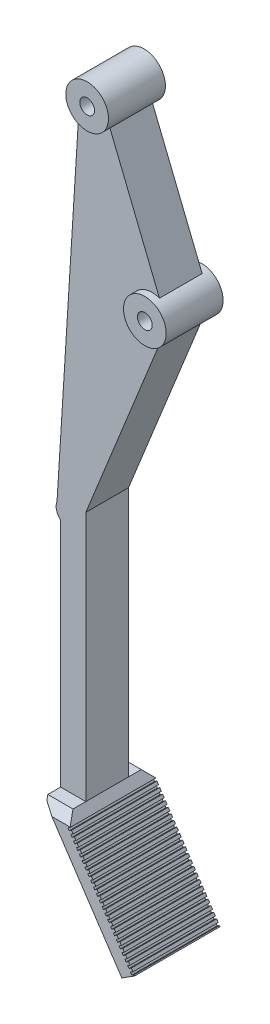
from build123d import *

# Parameters (mm, degrees)
SKETCH1_R            = 7.5
BOSS_EXTRUDE1_DEPTH  = 10
BOSS_EXTRUDE2_DEPTH  = 7.5
SKETCH3_R            = 2.6
CUT_EXTRUDE1_DEPTH   = 69.367154188
BOSS_EXTRUDE3_DEPTH  = 7.5
SKETCH6_R            = 7.5
BOSS_EXTRUDE4_DEPTH  = 10
SKETCH7_R            = 2.6
CUT_EXTRUDE2_DEPTH   = 139.291550533
BOSS_EXTRUDE8_DEPTH  = 7.5
SKETCH16_W           = 8.835752036
SKETCH16_H           = 88
BOSS_EXTRUDE9_DEPTH  = 7.5
BOSS_EXTRUDE10_DEPTH = 15
CHAMFER1_SIZE        = 3
CHAMFER2_SIZE        = 2
CUT_EXTRUDE3_DEPTH   = 259.435923483


with BuildPart() as part:
    # Sketch1 → Boss-Extrude1 (new, symmetric)
    with BuildSketch(Plane.XY):
        Circle(SKETCH1_R)
    extrude(amount=BOSS_EXTRUDE1_DEPTH, both=True)

    # Sketch2 → Boss-Extrude2 (add, symmetric)
    with BuildSketch(Plane.XY):
        with BuildLine():
            Line((5.502792208, -5.096006075), (24.97443042, -53.29000183))
            ThreePointArc((24.97443042, -53.29000183), (22.170934791, -59.894623641), (15.566312979, -57.091128012))
            Line((15.566312979, -57.091128012), (-5.395048503, -5.209937778))
            ThreePointArc((-5.395048503, -5.209937778), (0.078404622, -7.49959017), (5.502792208, -5.096006075))
        make_face()
    extrude(amount=BOSS_EXTRUDE2_DEPTH, both=True)

    # Sketch3 → Cut-Extrude1 (cut, through all)
    with BuildSketch(Plane.XY.offset(10)):
        Circle(SKETCH3_R)
    extrude(amount=-CUT_EXTRUDE1_DEPTH, mode=Mode.SUBTRACT)

    # Sketch5 → Boss-Extrude3 (add, symmetric)
    with BuildSketch(Plane.XY):
        with BuildLine():
            Line((15.566312979, -57.091128012), (-13.08078666, -127.995187718))
            ThreePointArc((-13.08078666, -127.995187718), (-10.670876789, -133.672579589), (-4.993484918, -131.262669718))
            Line((-4.993484918, -131.262669718), (24.944176558, -57.164357377))
            ThreePointArc((24.944176558, -57.164357377), (20.230755301, -60.263901008), (15.566312979, -57.091128012))
        make_face()
    extrude(amount=BOSS_EXTRUDE3_DEPTH, both=True)

    # Sketch6 → Boss-Extrude4 (add, symmetric)
    with BuildSketch(Plane.XY):
        with Locations((20.2703717, -55.190564921)):
            Circle(SKETCH6_R)
    extrude(amount=BOSS_EXTRUDE4_DEPTH, both=True)

    # Sketch7 → Cut-Extrude2 (cut, through all)
    with BuildSketch(Plane.XY.offset(10)):
        with Locations((20.2703717, -55.190564921)):
            Circle(SKETCH7_R)
    extrude(amount=-CUT_EXTRUDE2_DEPTH, mode=Mode.SUBTRACT)

    # Sketch11 → Boss-Extrude8 (add, symmetric)
    with BuildSketch(Plane.XY):
        with BuildLine():
            Line((-5.395048503, -5.209937778), (-13.08078666, -127.995187718))
            Line((-13.08078666, -127.995187718), (14.432076042, -59.898462945))
            ThreePointArc((14.432076042, -59.898462945), (12.821975428, -56.068854724), (13.497151784, -51.969774339))
            Line((13.497151784, -51.969774339), (-5.395048503, -5.209937778))
        make_face()
    extrude(amount=BOSS_EXTRUDE8_DEPTH, both=True)

    # Sketch16 → Boss-Extrude9 (add, symmetric)
    with BuildSketch(Plane.XY):
        with Locations((-7.390806842, -170.261622843)):
            Rectangle(SKETCH16_W, SKETCH16_H)
    extrude(amount=BOSS_EXTRUDE9_DEPTH, both=True)

    # Sketch17 → Boss-Extrude10 (add, symmetric)
    with BuildSketch(Plane(origin=(0, 0, 0), x_dir=(-1, 0, 0), z_dir=(0, 0, -1))):
        Polygon((11.80868286, -214.261622843), (2.972930824, -214.261622843), (-21.695736326, -251.232618801), (-15.495288767, -255.182156512), align=None)
    extrude(amount=BOSS_EXTRUDE10_DEPTH, both=True)

    # Chamfer1
    chamfer1_edges = [part.edges().sort_by_distance(p)[0] for p in [
        (-7.390806842, -214.261622843, 15),
        (-7.390806842, -214.261622843, -15),
    ]]
    chamfer(chamfer1_edges, length=CHAMFER1_SIZE)

    # Chamfer2
    chamfer2_edges = [part.edges().sort_by_distance(p)[0] for p in [
        (2.844168626, -236.221889677, 15),
        (2.844168626, -236.221889677, -15),
    ]]
    chamfer(chamfer2_edges, length=CHAMFER2_SIZE)

    # Sketch18 → Cut-Extrude3 (cut, through all)
    with BuildSketch(Plane.XY.offset(15)):
        Polygon((-0.922260896, -217.334967226), (-0.478234895, -218.000430155), (-1.310063556, -218.555462656), (-1.754089558, -217.889999727), align=None)
        Polygon((-0.755031055, -219.387291318), (0.076797607, -218.832258816), (0.520823608, -219.497721745), (-0.311005053, -220.052754247), align=None)
        Polygon((0.244027448, -220.884582909), (1.07585611, -220.329550407), (1.519882111, -220.995013336), (0.68805345, -221.550045838), align=None)
        Polygon((1.243085951, -222.381874499), (2.074914613, -221.826841998), (2.518940614, -222.492304927), (1.687111953, -223.047337429), align=None)
        Polygon((2.242144454, -223.87916609), (3.073973116, -223.324133588), (3.517999117, -223.989596518), (2.686170456, -224.544629019), align=None)
        Polygon((3.241202957, -225.376457681), (4.073031619, -224.821425179), (4.51705762, -225.486888108), (3.685228959, -226.04192061), align=None)
        Polygon((4.24026146, -226.873749271), (5.072090122, -226.31871677), (5.516116123, -226.984179699), (4.684287462, -227.539212201), align=None)
        Polygon((5.239319963, -228.371040862), (6.071148625, -227.81600836), (6.515174626, -228.48147129), (5.683345965, -229.036503791), align=None)
        Polygon((6.238378466, -229.868332453), (7.070207128, -229.313299951), (7.514233129, -229.97876288), (6.682404468, -230.533795382), align=None)
        Polygon((7.237436969, -231.365624043), (8.069265631, -230.810591542), (8.513291632, -231.476054471), (7.681462971, -232.031086973), align=None)
        Polygon((8.236495472, -232.862915634), (9.068324134, -232.307883132), (9.512350135, -232.973346062), (8.680521474, -233.528378563), align=None)
        Polygon((9.235553975, -234.360207225), (10.067382637, -233.805174723), (10.511408638, -234.470637652), (9.679579977, -235.025670154), align=None)
        Polygon((10.234612478, -235.857498816), (11.06644114, -235.302466314), (11.510467141, -235.967929243), (10.67863848, -236.522961745), align=None)
        Polygon((11.233670981, -237.354790406), (12.065499643, -236.799757905), (12.509525644, -237.465220834), (11.677696983, -238.020253335), align=None)
        Polygon((12.232729484, -238.852081997), (13.064558146, -238.297049495), (13.508584147, -238.962512424), (12.676755486, -239.517544926), align=None)
        Polygon((13.231787987, -240.349373588), (14.063616649, -239.794341086), (14.50764265, -240.459804015), (13.675813989, -241.014836517), align=None)
        Polygon((14.23084649, -241.846665178), (15.062675152, -241.291632677), (15.506701153, -241.957095606), (14.674872492, -242.512128108), align=None)
        Polygon((15.229904993, -243.343956769), (16.061733655, -242.788924267), (16.505759656, -243.454387197), (15.673930995, -244.009419698), align=None)
        Polygon((16.228963496, -244.84124836), (17.060792158, -244.286215858), (17.504818159, -244.951678787), (16.672989498, -245.506711289), align=None)
        Polygon((17.228021999, -246.33853995), (18.059850661, -245.783507449), (18.503876662, -246.448970378), (17.672048001, -247.00400288), align=None)
        Polygon((18.227080502, -247.835831541), (19.058909164, -247.280799039), (19.502935165, -247.946261969), (18.671106504, -248.50129447), align=None)
        Polygon((19.226139005, -249.333123132), (20.057967667, -248.77809063), (20.501993668, -249.443553559), (19.670165007, -249.998586061), align=None)
        Polygon((20.225197509, -250.830414722), (21.05702617, -250.275382221), (21.501052171, -250.94084515), (20.66922351, -251.495877652), align=None)
        Polygon((21.224256012, -252.327706313), (22.056084673, -251.772673811), (22.500110674, -252.438136741), (21.668282013, -252.993169242), align=None)
    extrude(amount=-CUT_EXTRUDE3_DEPTH, mode=Mode.SUBTRACT)


solid = part.part
